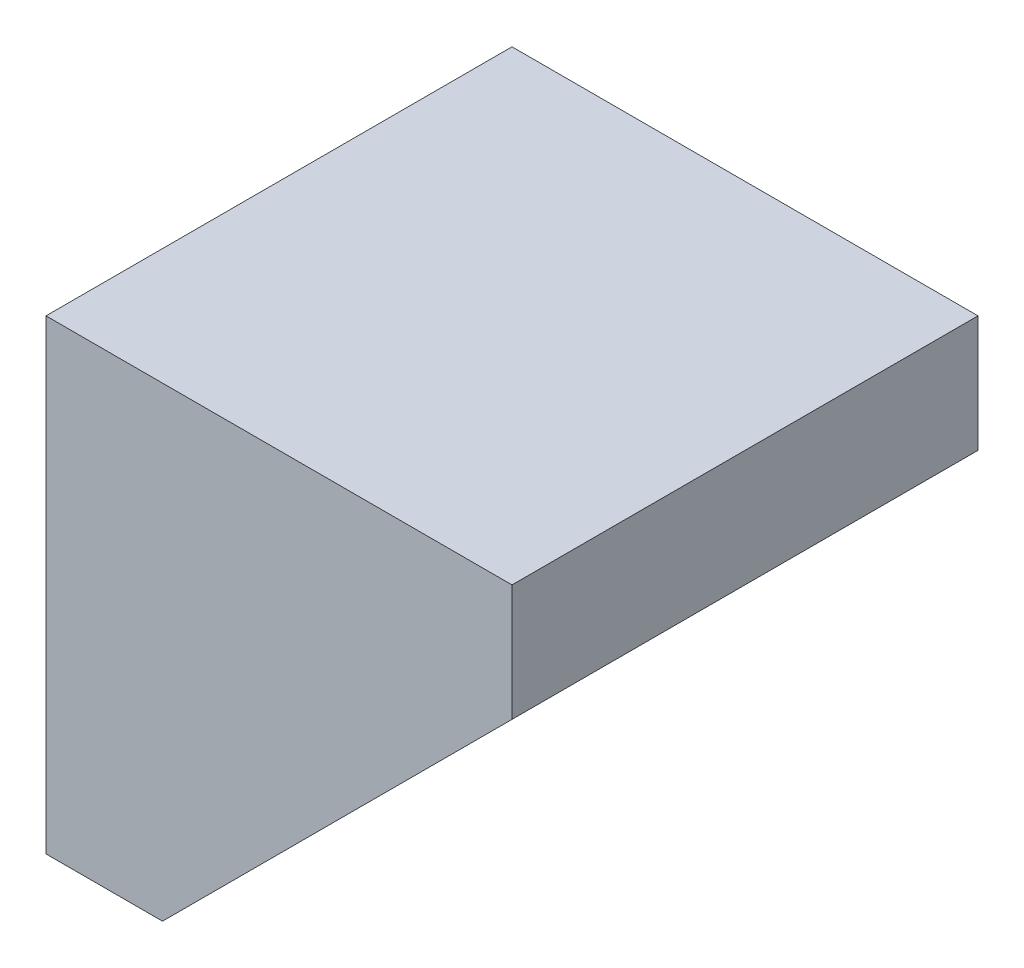
from build123d import *

# Parameters (mm, degrees)
SKETCH_1_W                = 80
SKETCH_1_H                = 80
EXTRUDE_1_DEPTH           = 80
HOLE_WIZARD_1_D           = 11
HOLE_WIZARD_1_CBORE_D     = 18
HOLE_WIZARD_1_CBORE_DEPTH = 50
CUT_EXTRUDE_1_DEPTH       = 121


with BuildPart() as part:
    # 草图1 → 凸台-拉伸1 (new body)
    with BuildSketch(Plane(origin=(0, 0, 0), x_dir=(0, 0, -1), z_dir=(1, 0, 0))):
        Rectangle(SKETCH_1_W, SKETCH_1_H)
    extrude(amount=EXTRUDE_1_DEPTH)

    # 打孔尺寸(%根据)内六角圆柱头螺钉的类型1 (through all)
    with Locations(Plane(origin=(80, 0, 0), x_dir=(0, 0, -1), z_dir=(1, 0, 0))):
        with Locations((-25, 0), (25, 0)):
            CounterBoreHole(HOLE_WIZARD_1_D / 2, HOLE_WIZARD_1_CBORE_D / 2, HOLE_WIZARD_1_CBORE_DEPTH)

    # 草图2 → 切除-拉伸1 (cut, through all)
    with BuildSketch(Plane.XY.offset(40)):
        Polygon((20, -40), (80, 20), (80, -40), align=None)
    extrude(amount=-CUT_EXTRUDE_1_DEPTH, mode=Mode.SUBTRACT)


solid = part.part
